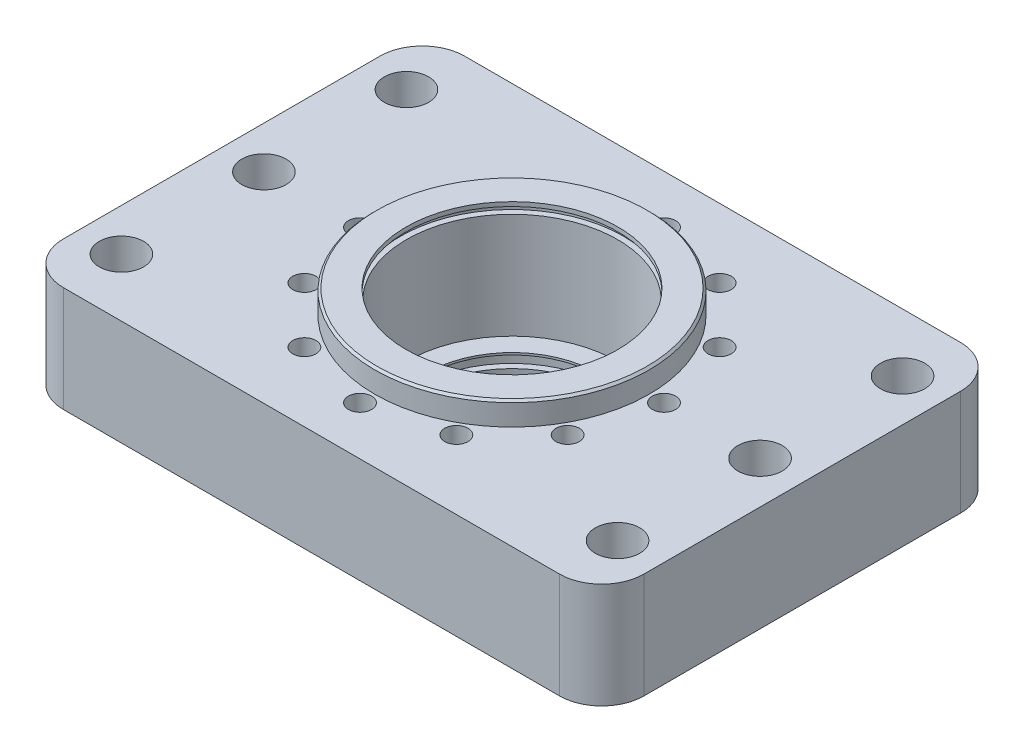
SolidWorks part; units mm, degrees
material "普通碳钢"
ref_plane "Front Plane" through (0, 0, 0) normal (0, 0, 1) x (1, 0, 0)
ref_plane "Top Plane" through (0, 0, 0) normal (0, 1, 0) x (1, 0, 0)
ref_plane "Right Plane" through (0, 0, 0) normal (1, 0, 0) x (0, 0, -1)
sketch "Sketch1" plane through (0, 0, 0) normal (0, 1, 0) x (1, 0, 0)
  circle A0 centre (0, 0) radius 102.5
  dimension "D1" = 205
extrude "Boss-Extrude1" add sketch "Sketch1" along normal blind 50
sketch "Sketch2" plane through (0, 50, 0) normal (0, 1, 0) x (1, 0, 0)
  circle A0 centre (0, 0) radius 65
  dimension "D1" = 130
extrude "Boss-Extrude2" add sketch "Sketch2" along normal blind 4
sketch "Sketch3" plane through (0, 0, 0) normal (0, -1, 0) x (1, 0, 0)
  circle A0 centre (0, 0) radius 75
  dimension "D1" = 150
extrude "Boss-Extrude3" add sketch "Sketch3" along normal blind 12
chamfer "Chamfer1" distance 1 angle 45 2 edges at (0, -12, -75) (0, 54, 65)
sketch "Sketch4" plane through (0, 54, 0) normal (0, 1, 0) x (1, 0, 0)
  circle A0 centre (0, 0) radius 50
  dimension "D1" = 100
extrude "Cut-Extrude1" cut sketch "Sketch4" against normal blind 55
sketch "Sketch5" plane through (0, -1, 0) normal (0, 1, 0) x (1, 0, 0)
  circle A0 centre (0, 0) radius 40.5
  dimension "D1" = 81
extrude "Cut-Extrude2" cut sketch "Sketch5" against normal through all
sketch "Sketch6" plane through (0, -12, 0) normal (0, -1, 0) x (1, 0, 0)
  circle A0 centre (0, 0) radius 45.5
  dimension "D1" = 91
extrude "Cut-Extrude3" cut sketch "Sketch6" against normal blind 7 from offset 3 offset against normal yes
sketch "Sketch7" plane through (0, -12, 0) normal (0, -1, 0) x (1, 0, 0)
  circle A0 centre (0, 0) radius 42.5
  dimension "D1" = 85
extrude "Cut-Extrude4" cut sketch "Sketch7" against normal blind 5
sketch "Sketch8" plane through (0, 54, 0) normal (0, 1, 0) x (1, 0, 0)
  circle A0 centre (0, 0) radius 52.75
  dimension "D1" = 105.5
extrude "Cut-Extrude5" cut sketch "Sketch8" against normal blind 3 from offset 2 offset against normal yes
sketch "Sketch9" plane through (0, 54, 0) normal (0, 1, 0) x (1, 0, 0)
  circle A0 centre (0, 0) radius 50.25
  dimension "D1" = 100.5
extrude "Cut-Extrude6" cut sketch "Sketch9" against normal blind 4
hole_wizard "Hole Size per Socket Head Cap Screw Type1" positions "Sketch11" profile "Sketch10" counterbore size "M10" standard "GB" end condition through all
sketch "Sketch11" plane through (0, -12, 0) normal (0, -1, 0) x (-1, 0, 0)
  point P0 (0, 72)
  dimension "D1" = 0
  dimension "D2" = 72
sketch "Sketch10" plane through (0, -12, -72) normal (1, 0, 0) x (0, 0, -1)
  line L0 (0, 0) -> (0, 66)
  line L1 (0, 66) -> (5.5, 66)
  line L3 (5.5, 66) -> (5.5, 33)
  line L4 (5.5, 33) -> (9, 33)
  line L5 (9, 33) -> (9, 0)
  line L7 (9, 0) -> (0, 0)
  line L11 (0, -6.35) -> (0, 107.95) construction
  dimension "通孔孔直径" = 11
  dimension "通孔孔深度" = 66
  dimension "柱形沉头孔直径" = 18
  dimension "柱形沉头孔深度" = 33
pattern_circular "CirPattern1" count 12 over 360 about axis through (0, 0, 0) along (0, 1, 0) of "Hole Size per Socket Head Cap Screw Type1"
sketch "Sketch14" plane through (0, 50, 0) normal (0, 1, 0) x (1, 0, 0)
  circle A0 centre (0, 0) radius 82.5
  dimension "D1" = 165
extrude "Cut-Extrude7" cut sketch "Sketch14" against normal blind 20 flip side to cut
chamfer "Chamfer4" distance 1.5 angle 45 2 edges at (0, 30, 102.5) (0, 0, 102.5)
sketch "Sketch17" plane through (0, 30, 0) normal (0, 1, 0) x (1, 0, 0)
  line L0 (0, 0) -> (122.9816, 0) construction
  line L1 (0, 0) -> (92.5, 0) construction
  circle A0 centre (92.5, 0) radius 5.5
  dimension "D1" = 11
  dimension "D2" = 92.5
  dimension "D3" = 0
extrude "Cut-Extrude11" cut sketch "Sketch17" against normal through all
pattern_circular "CirPattern4" count 10 over 360 about axis through (0, 0, 0) along (0, 1, 0) of "Cut-Extrude11"
sketch "Sketch18" plane through (0, 0, 0) normal (0, -1, 0) x (1, 0, 0)
  line L0 (0, 0) -> (87.9727, -28.5841) construction
  line L1 (0, 0) -> (136.2228, 0) construction
  circle A0 centre (87.9727, -28.5841) radius 6
  dimension "D1" = 12
  dimension "D2" = 92.5
  dimension "D3" = 18
hole_wizard "M12 Tapped Hole1" positions "Sketch19" profile "Sketch21" tap size "M12" standard "GB" end condition through all
sketch "Sketch19" plane through (0, 0, 0) normal (0, -1, 0) x (-1, 0, 0)
  point P0 (-87.9727, 28.5841)
sketch "Sketch21" plane through (87.9727, 0, -28.5841) normal (1, 0, 0) x (0, 0, -1)
  line L0 (0, 0) -> (0, 54)
  line L1 (0, 54) -> (5.1, 54)
  line L2 (5.1, 54) -> (5.1, 0)
  line L5 (5.1, 0) -> (0, 0)
  line L11 (0, -6.35) -> (0, 107.95) construction
  dimension "通孔螺纹孔钻头直径" = 10.2
  dimension "通孔螺纹孔钻头深度" = 54
cosmetic thread "Cosmetic Thread2" parameters "D2"=12
sketch "Sketch22" plane through (0, 0, 0) normal (0, -1, 0) x (1, 0, 0)
  circle A0 centre (0, 0) radius 82.5
  dimension "D1" = 165
extrude "Cut-Extrude12" cut sketch "Sketch22" against normal through all flip side to cut
sketch "Sketch24" plane through (0, 0, 0) normal (0, -1, 0) x (1, 0, 0)
  line L1 (137.5, -95) -> (-137.5, -95)
  line L2 (137.5, -95) -> (137.5, 95)
  line L3 (137.5, 95) -> (-137.5, 95)
  line L4 (-137.5, -95) -> (-137.5, 95)
  line L5 (137.5, -95) -> (-137.5, 95) construction
  line L6 (137.5, 95) -> (-137.5, -95) construction
  circle A0 centre (0, 0) radius 82.5
  dimension "D1" = 275
  dimension "D2" = 190
extrude "Boss-Extrude4" add sketch "Sketch24" against normal up to surface (50 mm away) up to face at (0, 50, 65)
fillet "Fillet1" radius 20 4 edges at (-137.5, 25, -95) (137.5, 25, -95) (137.5, 25, 95) (-137.5, 25, 95)
other "Move Face1" face at (0, 0, 0) parameters "D1"=7
other "Move Face2" face at (0, 50, 65) parameters "D1"=7
hole_wizard "Ø21.0 (21) Diameter Hole1" positions "Sketch25" profile "Sketch26" hole size "Ø21.0" standard "GB" end condition through all
sketch "Sketch25" plane through (0, -7, 0) normal (0, -1, 0) x (-1, 0, 0)
  line L0 (0, 0) -> (-187.8964, 0) construction
  line L2 (0, 0) -> (0, 129.1744) construction
  point P0 (-117.5, 67.5)
  point P2 (-117.5, 0)
  point P4 (-117.5, -67.5)
  point P6 (117.5, 67.5)
  point P8 (117.5, 0)
  point P10 (117.5, -67.5)
  dimension "D1" = 235
  dimension "D2" = 135
sketch "Sketch26" plane through (117.5, -7, -67.5) normal (1, 0, 0) x (0, 0, -1)
  line L0 (0, 0) -> (0, 61)
  line L1 (0, 61) -> (10.5, 61)
  line L2 (10.5, 61) -> (10.5, 0)
  line L5 (10.5, 0) -> (0, 0)
  line L11 (0, -6.35) -> (0, 107.95) construction
  dimension "通孔孔直径" = 21
  dimension "通孔孔深度" = 61
